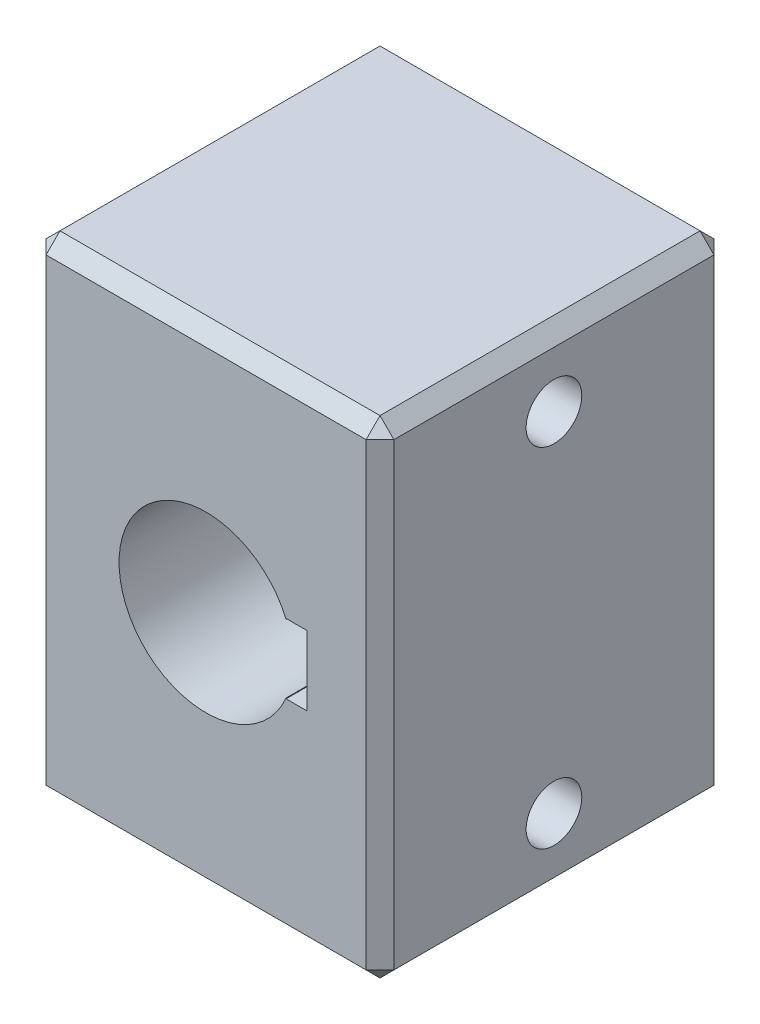
from build123d import *

# Parameters (mm, degrees)
SKETCH_1_W          = 50
SKETCH_1_H          = 70
EXTRUDE_1_DEPTH     = 50
SKETCH_2_R          = 12.5
CUT_EXTRUDE_1_DEPTH = 66.954529791
SKETCH_12_R         = 4
CUT_EXTRUDE_5_DEPTH = 58
CHAMFER_1_SIZE      = 2
CUT_EXTRUDE_START   = -13.5
CUT_EXTRUDE_6_DEPTH = 3


with BuildPart() as part:
    # 草图1 → 凸台-拉伸1 (new body)
    with BuildSketch(Plane.XY):
        Rectangle(SKETCH_1_W, SKETCH_1_H)
    extrude(amount=EXTRUDE_1_DEPTH)

    # 草图2 → 切除-拉伸1 (cut, through all)
    with BuildSketch(Plane.XY.offset(50)):
        Circle(SKETCH_2_R)
    extrude(amount=-CUT_EXTRUDE_1_DEPTH, mode=Mode.SUBTRACT)

    # 草图12 → 切除-拉伸5 (cut)
    with BuildSketch(Plane(origin=(25, 0, 0), x_dir=(0, 0, -1), z_dir=(1, 0, 0))):
        with Locations((-25, 25)):
            Circle(SKETCH_12_R)
    cut_extrude_5 = extrude(amount=-CUT_EXTRUDE_5_DEPTH, mode=Mode.SUBTRACT)

    # 镜向1: 切除-拉伸5 across plane
    add(cut_extrude_5.mirror(Plane.ZX), mode=Mode.SUBTRACT)

    # 倒角1
    chamfer_1_edges = [part.edges().sort_by_distance(p)[0] for p in [
        (-25, 0, 50),
        (0, -35, 50),
        (25, 0, 50),
        (0, -35, 0),
        (-25, 0, 0),
        (0, 35, 0),
        (25, 0, 0),
        (25, -35, 25),
        (-25, -35, 25),
        (-25, 35, 25),
        (25, 35, 25),
        (0, 35, 50),
    ]]
    chamfer(chamfer_1_edges, length=CHAMFER_1_SIZE)

    # 草图13 → 切除-拉伸6 (cut)
    with BuildSketch(Plane(origin=(25, 0, 0), x_dir=(0, 0, -1), z_dir=(1, 0, 0)).offset(CUT_EXTRUDE_START)):
        with BuildLine():
            Line((-50, 5), (-28, 5))
            ThreePointArc((-28, 5), (-23, 0), (-28, -5))
            Line((-28, -5), (-50, -5))
            ThreePointArc((-50, -5), (-55, 0), (-50, 5))
        make_face()
    extrude(amount=CUT_EXTRUDE_6_DEPTH, mode=Mode.SUBTRACT)


solid = part.part
